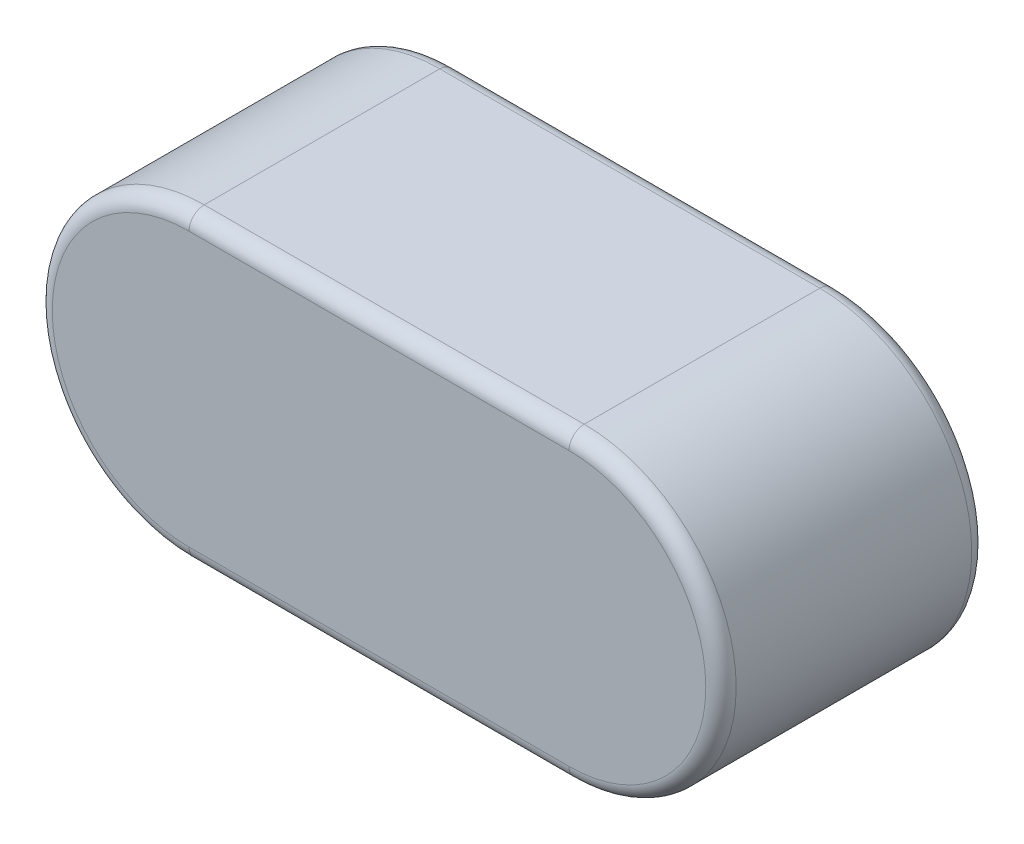
from build123d import *

# Parameters (mm, degrees)
EXTRUDE_523_DEPTH = 7
FILLET_1_R        = 0.4


with BuildPart() as part:
    # 草图1 → Extrude 523 (new body)
    with BuildSketch(Plane.XY):
        with BuildLine():
            Line((-5, 4), (5, 4))
            ThreePointArc((5, 4), (9, 0), (5, -4))
            Line((5, -4), (-5, -4))
            ThreePointArc((-5, -4), (-9, 0), (-5, 4))
        make_face()
    extrude(amount=EXTRUDE_523_DEPTH)

    # 圆角1
    fillet_1_edges = [part.edges().sort_by_distance(p)[0] for p in [
        (9, 0, 7),
        (0, 4, 7),
        (-9, 0, 7),
        (0, 4, 0),
        (9, 0, 0),
        (0, -4, 0),
        (-9, 0, 0),
        (0, -4, 7),
    ]]
    fillet(fillet_1_edges, radius=FILLET_1_R)


solid = part.part
